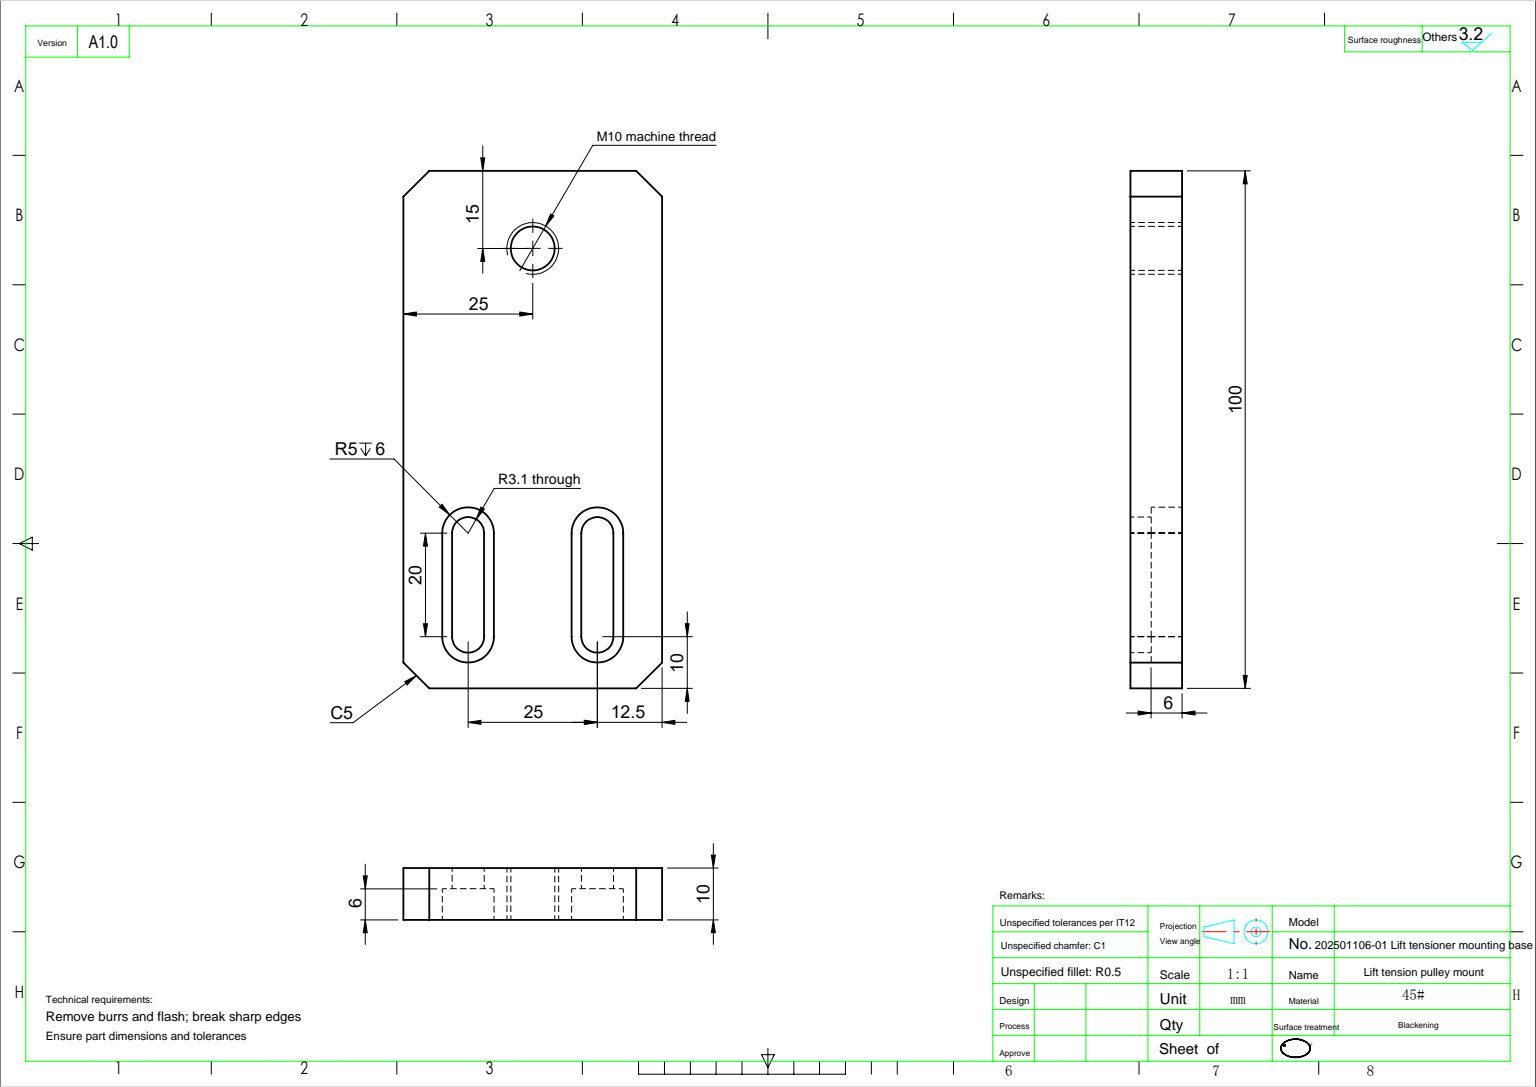
SolidWorks part; units mm, degrees
ref_plane "前视基准面" through (0, 0, 0) normal (0, 0, 1) x (1, 0, 0)
ref_plane "上视基准面" through (0, 0, 0) normal (0, 1, 0) x (1, 0, 0)
ref_plane "右视基准面" through (0, 0, 0) normal (1, 0, 0) x (0, 0, -1)
sketch "草图1" plane through (0, 0, 0) normal (0, 0, 1) x (1, 0, 0)
  line L1 (-25, 50) -> (25, 50)
  line L2 (-25, 50) -> (-25, -50)
  line L3 (-25, -50) -> (25, -50)
  line L4 (25, 50) -> (25, -50)
  line L5 (0, -50) -> (0, 50) construction
  line L6 (-25, 0) -> (25, 0) construction
  point P0 (0, 0)
  dimension "D1" = 50
  dimension "D2" = 100
extrude "凸台-拉伸1" add sketch "草图1" along normal blind 10
sketch "草图2" plane through (0, 0, 10) normal (0, 0, 1) x (1, 0, 0)
  line L0 (-12.5, -20) -> (-12.5, -40) construction
  line L1 (-9.4, -20) -> (-9.4, -40)
  line L2 (-15.6, -20) -> (-15.6, -40)
  line L3 (12.5, -40) -> (12.5, -20) construction
  line L4 (9.4, -40) -> (9.4, -20)
  line L5 (15.6, -40) -> (15.6, -20)
  line L7 (-25, 50) -> (-25, -50) construction
  line L9 (-25, -50) -> (25, -50) construction
  arc A0 (-9.4, -20) -> (-15.6, -20) centre (-12.5, -20) ccw
  arc A1 (-15.6, -40) -> (-9.4, -40) centre (-12.5, -40) ccw
  arc A2 (9.4, -40) -> (15.6, -40) centre (12.5, -40) ccw
  arc A3 (15.6, -20) -> (9.4, -20) centre (12.5, -20) ccw
  point P2 (-12.5, -30)
  point P9 (12.5, -30)
  dimension "D2" = 3.1
  dimension "D3" = 25
  dimension "D1" = 20
  dimension "D4" = 12.5
  dimension "D5" = 10
extrude "切除-拉伸1" cut sketch "草图2" against normal blind 10
sketch "草图3" plane through (0, 0, 10) normal (0, 0, 1) x (1, 0, 0)
  line L0 (-12.5, -20) -> (-12.5, -40) construction
  line L1 (-7.5, -20) -> (-7.5, -40)
  line L2 (-17.5, -20) -> (-17.5, -40)
  line L3 (12.5, -20) -> (12.5, -40) construction
  line L4 (17.5, -20) -> (17.5, -40)
  line L5 (7.5, -20) -> (7.5, -40)
  line L6 (-25, -50) -> (25, -50) construction
  arc A0 (-7.5, -20) -> (-17.5, -20) centre (-12.5, -20) ccw
  arc A1 (-17.5, -40) -> (-7.5, -40) centre (-12.5, -40) ccw
  arc A2 (17.5, -20) -> (7.5, -20) centre (12.5, -20) ccw
  arc A3 (7.5, -40) -> (17.5, -40) centre (12.5, -40) ccw
  point P2 (-12.5, -30)
  point P10 (12.5, -30)
  dimension "D2" = 5
  dimension "D1" = 20
  dimension "D3" = 10
extrude "切除-拉伸2" cut sketch "草图3" against normal blind 6
chamfer "倒角1" distance 5 angle 45 4 edges at (25, 50, 5) (-25, 50, 5) (25, -50, 5) (-25, -50, 5)
sketch "草图4" plane through (0, 0, 10) normal (0, 0, 1) x (1, 0, 0)
  line L0 (20, 50) -> (-20, 50) construction
  circle A0 centre (0, 35) radius 4.25
  point P4 (0, 0)
  dimension "D1" = 8.5
  dimension "D2" = 15
extrude "切除-拉伸3" cut sketch "草图4" against normal blind 10
cosmetic thread "装饰螺纹线1" parameters "D2"=10
